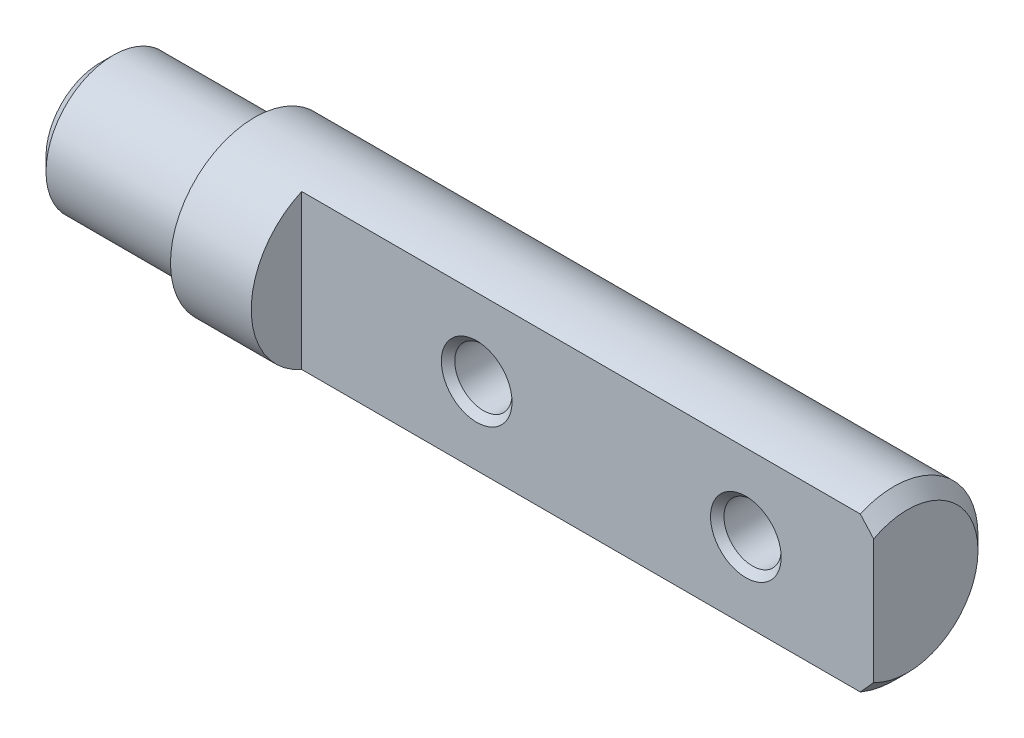
SolidWorks part; units mm, degrees
material "1023 碳钢板 (SS)"
ref_plane "前视" through (0, 0, 0) normal (0, 0, 1) x (1, 0, 0)
ref_plane "上视" through (0, 0, 0) normal (0, 1, 0) x (1, 0, 0)
ref_plane "右视" through (0, 0, 0) normal (1, 0, 0) x (0, 0, -1)
sketch "草图1" plane through (0, 0, 0) normal (0, 0, 1) x (1, 0, 0)
  line L0 (0, 0) -> (0, 10)
  line L1 (0, 10) -> (23, 10)
  line L2 (23, 12.5) -> (23, 10)
  line L5 (23, 12.5) -> (120, 12.5)
  line L6 (120, 12.5) -> (120, 0)
  line L7 (120, 0) -> (0, 0)
  dimension "D1" = 10
  dimension "D2" = 23
  dimension "D3" = 12.5
  dimension "D6" = 120
revolve "旋转2" add sketch "草图1" angle 360 about L7
chamfer "倒角1" distance 2 angle 45 2 edges at (120, 12.5, 0) (0, 10, 0)
sketch "草图2" plane through (0, 0, 0) normal (0, 1, 0) x (1, 0, 0)
  line L0 (118, 0) -> (125.1757, 0) construction
  line L1 (35, -5) -> (126.6245, -5)
  line L2 (35, -5) -> (35, -30.7679)
  line L3 (35, -30.7679) -> (126.6245, -30.7679)
  line L4 (126.6245, -5) -> (126.6245, -30.7679)
  line L5 (118, 12.5) -> (118, -12.5) construction
  line L6 (120, -10.5) -> (120, 10.5) construction
  dimension "D1" = 85
  dimension "D2" = 5
extrude "切除-拉伸1" cut sketch "草图2" against normal blind 20 and the other way blind 31
sketch "草图3" plane through (0, 0, 5) normal (0, 0, 1) x (1, 0, 0)
  line L0 (35, 0) -> (61, 0) construction
  line L1 (35, -11.4564) -> (35, 11.4564) construction
  line L2 (61, 0) -> (101, 0) construction
  dimension "D1" = 26
  dimension "D2" = 40
hole_wizard "M10 螺纹孔1" positions "草图5" profile "草图4" tap size "M10" standard "Gb"
sketch "草图5" plane through (0, 0, 5) normal (0, 0, 1) x (1, 0, 0)
  point P0 (61, 0)
  point P3 (101, 0)
sketch "草图4" plane through (61, 0, 5) normal (1, 0, 0) x (0, -1, 0)
  line L0 (0, 0) -> (0, 30.0537)
  line L1 (0, 30.0537) -> (4.25, 27.5)
  line L2 (4.25, 27.5) -> (4.25, 0)
  line L5 (4.25, 0) -> (0, 0)
  line L10 (0, 30.0537) -> (-4.25, 27.5) construction
  line L11 (0, -6.35) -> (0, 107.95) construction
  dimension "螺纹孔钻头直径" = 8.5
  dimension "螺纹孔钻头深度" = 27.5
  dimension "导头角度" = 118
cosmetic thread "孔螺蚊线1" parameters "D1"=17.5, "D2"=10
cosmetic thread "孔螺蚊线2" parameters "D1"=17.5, "D2"=10
chamfer "倒角3" distance 1 angle 45 2 edges at (105.25, 0, 5) (65.25, 0, 5)
